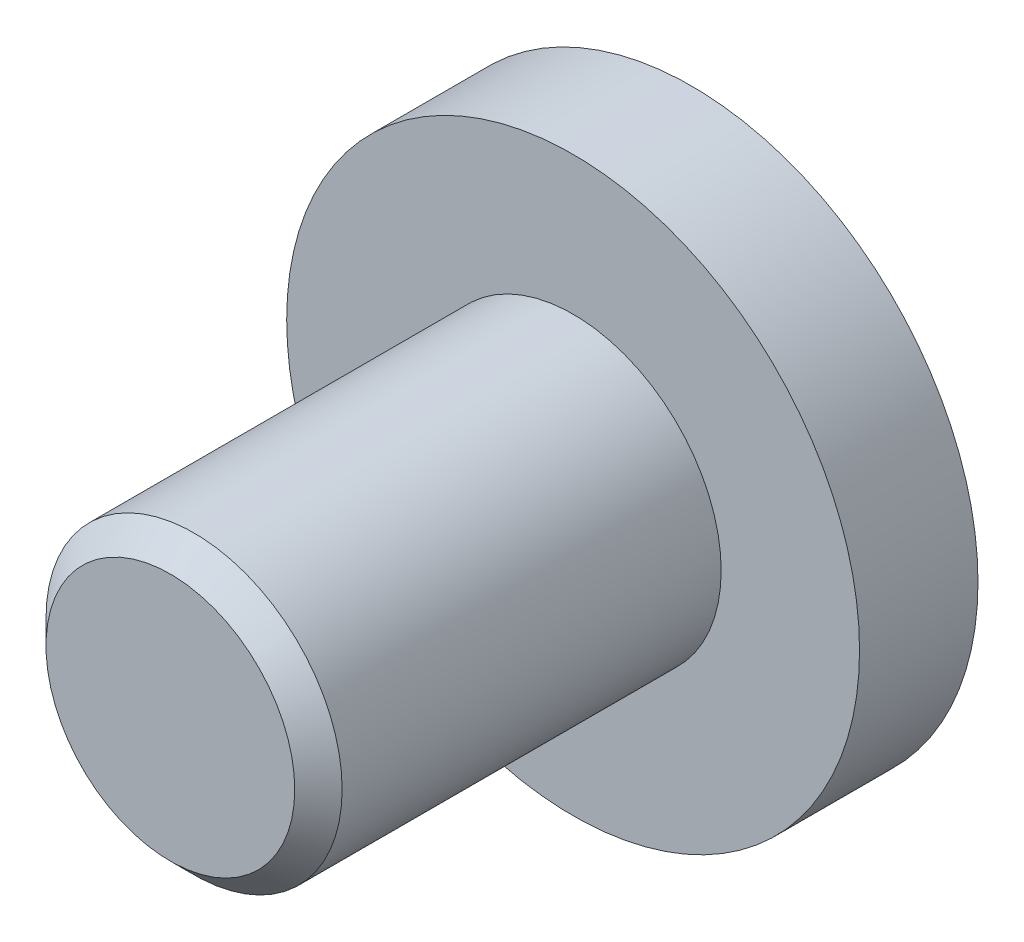
from build123d import *

# Parameters (mm, degrees)
SKETCH1_R           = 12.090742714
BOSS_EXTRUDE1_DEPTH = 5
SKETCH2_R           = 6.25
BOSS_EXTRUDE2_DEPTH = 17
CHAMFER1_SIZE       = 1


with BuildPart() as part:
    # Sketch1 → Boss-Extrude1 (new body)
    with BuildSketch(Plane.XY):
        Circle(SKETCH1_R)
    extrude(amount=BOSS_EXTRUDE1_DEPTH)

    # Sketch2 → Boss-Extrude2 (add)
    with BuildSketch(Plane.XY.offset(5)):
        Circle(SKETCH2_R)
    extrude(amount=BOSS_EXTRUDE2_DEPTH)

    # Chamfer1
    chamfer1_edges = [part.edges().sort_by_distance(p)[0] for p in [
        (-6.25, 0, 22),
    ]]
    chamfer(chamfer1_edges, length=CHAMFER1_SIZE)


solid = part.part
